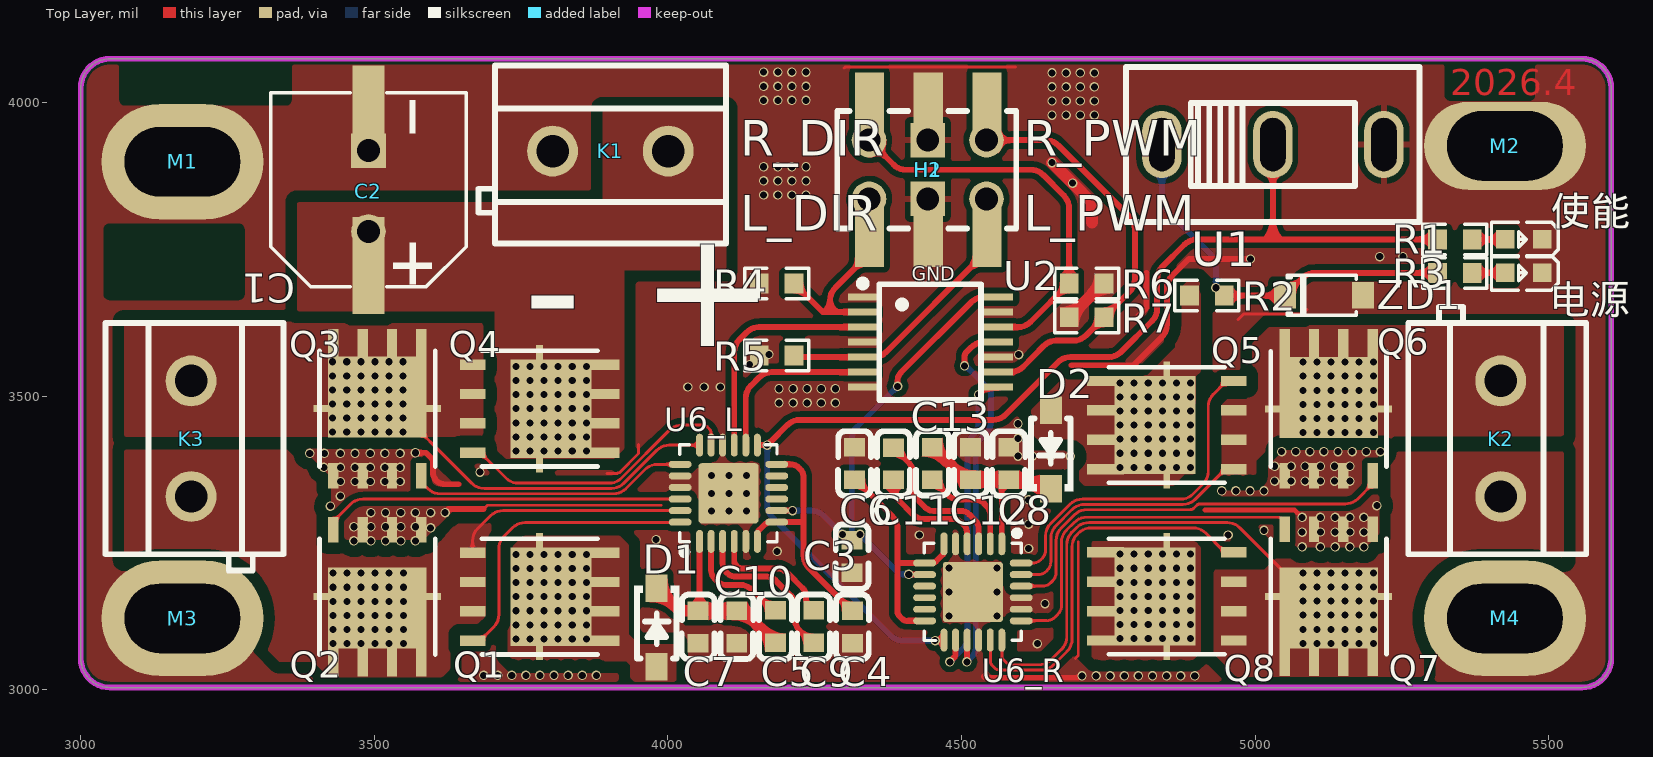
[diagram p0: Top Layer view]
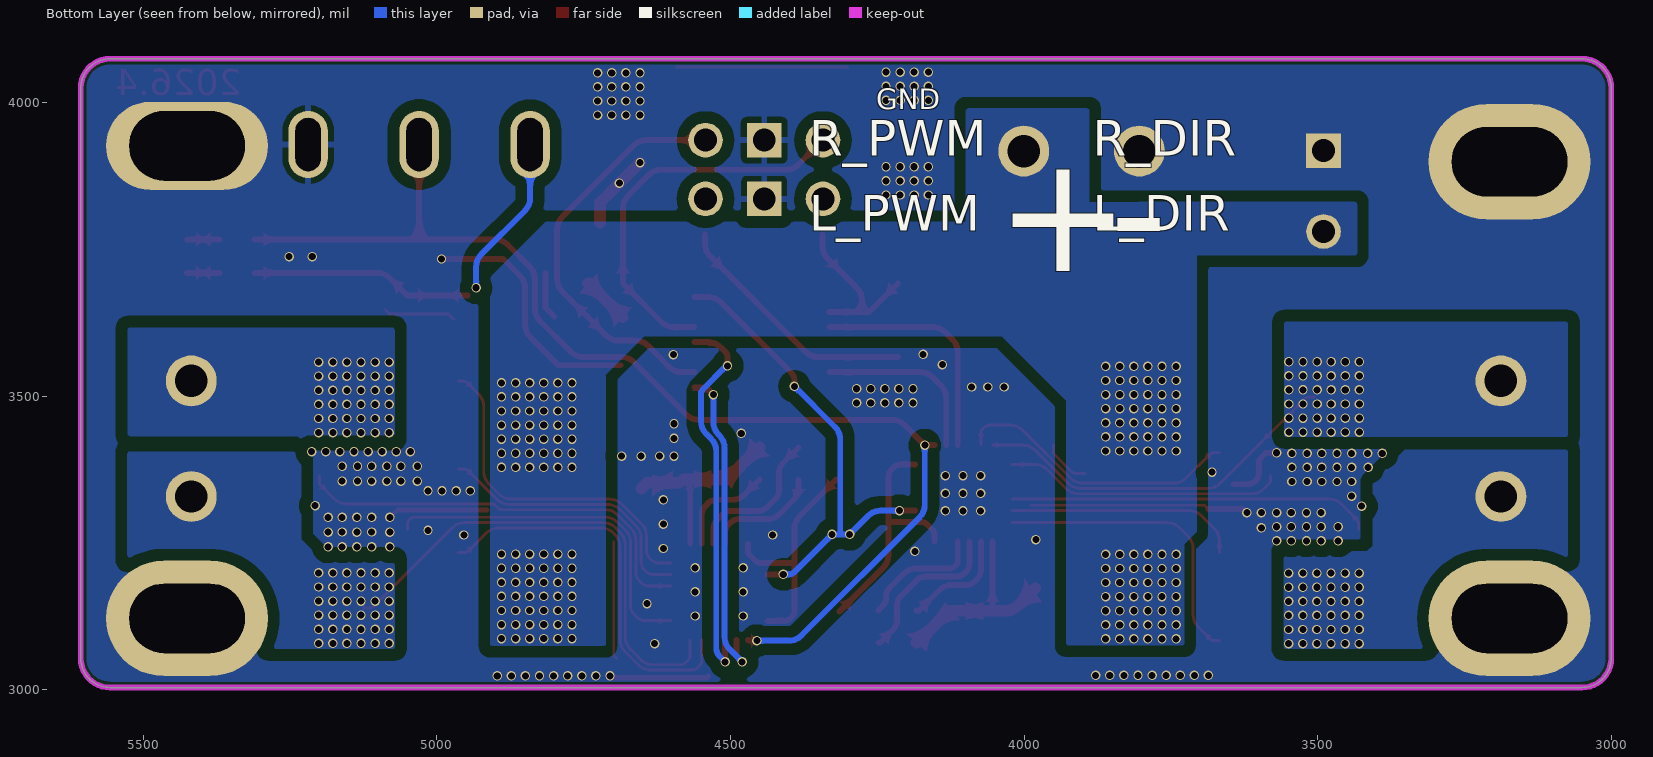
[diagram p1: Bottom Layer view, seen from below]
# Altium PCB MISC49921.pcbdoc (part 1 of 2)
Units mil, origin at the board's own origin, x right, y up, seen from the top; angles counter-clockwise.
Board outline 2606.3 x 1070.87 mil, 2 copper layers (Top Layer, Bottom Layer), stack 62.206 mil thick; 46 components, 37 nets, 219 pads, 514 vias.

## Layer stack, top to bottom
Top Solder Mask Layer: solder mask 0.394, Dk 3.3
Top Layer: signal copper 1.379
Dielectric1: surface 59.449, FR4, Dk 4.5
Bottom Layer: signal copper 1.378
Bottom Solder Mask Layer: solder mask 0.394, Dk 3.3

## Board outline
3050,4074.6 ccw(c3050,4024.6) 3000,4024.6 3000,3053.73 ccw(c3050,3053.73) 3050,3003.73 5556.3,3003.73 ccw(c5556.3,3053.73) 5606.3,3053.73 5606.3,4024.6 ccw(c5556.3,4024.6) 5556.3,4074.6

## Design rules (kind name [scope] priority, off if disabled: settings)
BoardOutlineClearance copperThickness2oz_1 [All] p2 off: genericclearance=8 ignorepadtopadclearanceinfootprint=FALSE except(0: Arc-SplitContinuation Track-SplitContinuation SMDPad-SplitContinuation THPad-SplitContinuation Via-SplitContinuation Fill-SplitContinuation Region-SplitContinuation Poly-SplitContinuation Text-SplitContinuation Hole-SplitContinuation; 6: Arc-CutoutEdge Track-CutoutEdge SMDPad-CutoutEdge THPad-CutoutEdge Via-CutoutEdge Text-CutoutEdge; 6.9: Hole-OutlineEdge Hole-CutoutEdge; 10: Poly-OutlineEdge Poly-CutoutEdge; 11.8: Arc-OutlineEdge Track-OutlineEdge SMDPad-OutlineEdge THPad-OutlineEdge Via-OutlineEdge Fill-OutlineEdge Region-OutlineEdge Text-OutlineEdge Fill-CutoutEdge Region-CutoutEdge)
BoardOutlineClearance Plane_innerPlane_1 [All] p4 off: genericclearance=4 ignorepadtopadclearanceinfootprint=FALSE except(0: Arc-SplitContinuation Track-SplitContinuation SMDPad-SplitContinuation THPad-SplitContinuation Via-SplitContinuation Fill-SplitContinuation Region-SplitContinuation Poly-SplitContinuation Text-SplitContinuation Hole-SplitContinuation; 6: Arc-CutoutEdge Track-CutoutEdge SMDPad-CutoutEdge THPad-CutoutEdge Via-CutoutEdge Text-CutoutEdge; 6.9: Hole-OutlineEdge Hole-CutoutEdge; 10: Poly-OutlineEdge Poly-CutoutEdge; 11.8: Arc-OutlineEdge Track-OutlineEdge SMDPad-OutlineEdge THPad-OutlineEdge Via-OutlineEdge Fill-OutlineEdge Region-OutlineEdge Text-OutlineEdge Fill-CutoutEdge Region-CutoutEdge)
BoardOutlineClearance Copper_copperRegion_1 [All] p6 off: genericclearance=4 ignorepadtopadclearanceinfootprint=FALSE except(0: Arc-SplitContinuation Track-SplitContinuation SMDPad-SplitContinuation THPad-SplitContinuation Via-SplitContinuation Fill-SplitContinuation Region-SplitContinuation Poly-SplitContinuation Text-SplitContinuation Hole-SplitContinuation; 6: Arc-CutoutEdge Track-CutoutEdge SMDPad-CutoutEdge THPad-CutoutEdge Via-CutoutEdge Text-CutoutEdge; 6.9: Hole-OutlineEdge Hole-CutoutEdge; 10: Poly-OutlineEdge Poly-CutoutEdge; 11.8: Arc-OutlineEdge Track-OutlineEdge SMDPad-OutlineEdge THPad-OutlineEdge Via-OutlineEdge Fill-OutlineEdge Region-OutlineEdge Text-OutlineEdge Fill-CutoutEdge Region-CutoutEdge)
BoardOutlineClearance Copper_直连_1 [All] p8 off: genericclearance=4 ignorepadtopadclearanceinfootprint=FALSE except(0: Arc-SplitContinuation Track-SplitContinuation SMDPad-SplitContinuation THPad-SplitContinuation Via-SplitContinuation Fill-SplitContinuation Region-SplitContinuation Poly-SplitContinuation Text-SplitContinuation Hole-SplitContinuation; 6: Arc-CutoutEdge Track-CutoutEdge SMDPad-CutoutEdge THPad-CutoutEdge Via-CutoutEdge Text-CutoutEdge; 6.9: Hole-OutlineEdge Hole-CutoutEdge; 10: Poly-OutlineEdge Poly-CutoutEdge; 11.8: Arc-OutlineEdge Track-OutlineEdge SMDPad-OutlineEdge THPad-OutlineEdge Via-OutlineEdge Fill-OutlineEdge Region-OutlineEdge Text-OutlineEdge Fill-CutoutEdge Region-CutoutEdge)
BoardOutlineClearance Copper_18_1 [All] p10 off: genericclearance=4 ignorepadtopadclearanceinfootprint=FALSE except(0: Arc-SplitContinuation Track-SplitContinuation SMDPad-SplitContinuation THPad-SplitContinuation Via-SplitContinuation Fill-SplitContinuation Region-SplitContinuation Poly-SplitContinuation Text-SplitContinuation Hole-SplitContinuation; 6: Arc-CutoutEdge Track-CutoutEdge SMDPad-CutoutEdge THPad-CutoutEdge Via-CutoutEdge Text-CutoutEdge; 6.9: Hole-OutlineEdge Hole-CutoutEdge; 10: Poly-OutlineEdge Poly-CutoutEdge; 11.8: Arc-OutlineEdge Track-OutlineEdge SMDPad-OutlineEdge THPad-OutlineEdge Via-OutlineEdge Fill-OutlineEdge Region-OutlineEdge Text-OutlineEdge Fill-CutoutEdge Region-CutoutEdge)
BoardOutlineClearance copperThickness1oz_1 [All] p12: genericclearance=4 ignorepadtopadclearanceinfootprint=FALSE except(0: Arc-SplitContinuation Track-SplitContinuation SMDPad-SplitContinuation THPad-SplitContinuation Via-SplitContinuation Fill-SplitContinuation Region-SplitContinuation Poly-SplitContinuation Text-SplitContinuation Hole-SplitContinuation; 6: Arc-CutoutEdge Track-CutoutEdge SMDPad-CutoutEdge THPad-CutoutEdge Via-CutoutEdge Text-CutoutEdge; 6.9: Hole-OutlineEdge Hole-CutoutEdge; 10: Poly-OutlineEdge Poly-CutoutEdge; 11.8: Arc-OutlineEdge Track-OutlineEdge SMDPad-OutlineEdge THPad-OutlineEdge Via-OutlineEdge Fill-OutlineEdge Region-OutlineEdge Text-OutlineEdge Fill-CutoutEdge Region-CutoutEdge)
Clearance copperThickness2oz [All] p1 off: gap=8 ignorepadtopadclearanceinfootprint=FALSE except(6: SMDPad-Track SMDPad-SMDPad THPad-Track SMDPad-THPad THPad-THPad Track-Via SMDPad-Via THPad-Via Via-Via Fill-SMDPad Region-SMDPad Fill-THPad Region-THPad Fill-Via Region-Via Arc-Track Arc-SMDPad Arc-THPad Arc-Via Fill-Arc Region-Arc Arc-Arc Text-Track SMDPad-Text Text-THPad Text-Via Fill-Text Region-Text Arc-Text Text-Text; 6.9: Hole-Track Hole-SMDPad Hole-THPad Hole-Via Fill-Hole Region-Hole Hole-Arc Hole-Text; 10: Poly-Track Poly-SMDPad Poly-THPad Poly-Via Poly-Fill Poly-Region Poly-Poly Poly-Arc Poly-Text Poly-Hole; 11.8: Fill-Track Region-Track; 20: Fill-Fill Fill-Region Region-Region)
Clearance Plane_innerPlane [All] p3 off: gap=4 ignorepadtopadclearanceinfootprint=FALSE except(6: SMDPad-Track SMDPad-SMDPad THPad-Track SMDPad-THPad THPad-THPad Track-Via SMDPad-Via THPad-Via Via-Via Fill-SMDPad Region-SMDPad Fill-THPad Region-THPad Fill-Via Region-Via Arc-Track Arc-SMDPad Arc-THPad Arc-Via Fill-Arc Region-Arc Arc-Arc Text-Track SMDPad-Text Text-THPad Text-Via Fill-Text Region-Text Arc-Text Text-Text; 6.9: Hole-Track Hole-SMDPad Hole-THPad Hole-Via Fill-Hole Region-Hole Hole-Arc Hole-Text; 10: Poly-Track Poly-SMDPad Poly-THPad Poly-Via Poly-Fill Poly-Region Poly-Poly Poly-Arc Poly-Text Poly-Hole; 11.8: Fill-Track Region-Track; 12: Fill-Fill Fill-Region Region-Region)
Clearance Copper_copperRegion [All] p5 off: gap=4 ignorepadtopadclearanceinfootprint=FALSE except(6: SMDPad-Track SMDPad-SMDPad THPad-Track SMDPad-THPad THPad-THPad Track-Via SMDPad-Via THPad-Via Via-Via Fill-SMDPad Region-SMDPad Fill-THPad Region-THPad Fill-Via Region-Via Arc-Track Arc-SMDPad Arc-THPad Arc-Via Fill-Arc Region-Arc Arc-Arc Text-Track SMDPad-Text Text-THPad Text-Via Fill-Text Region-Text Arc-Text Text-Text; 6.9: Hole-Track Hole-SMDPad Hole-THPad Hole-Via Fill-Hole Region-Hole Hole-Arc Hole-Text; 10: Poly-Track Poly-SMDPad Poly-THPad Poly-Via Poly-Fill Poly-Region Poly-Poly Poly-Arc Poly-Text Poly-Hole; 11.8: Fill-Track Region-Track; 12: Fill-Fill Fill-Region Region-Region)
Clearance Copper_直连 [All] p7 off: gap=4 ignorepadtopadclearanceinfootprint=FALSE except(6: SMDPad-Track SMDPad-SMDPad THPad-Track SMDPad-THPad THPad-THPad Track-Via SMDPad-Via THPad-Via Via-Via Fill-SMDPad Region-SMDPad Fill-THPad Region-THPad Fill-Via Region-Via Arc-Track Arc-SMDPad Arc-THPad Arc-Via Fill-Arc Region-Arc Arc-Arc Text-Track SMDPad-Text Text-THPad Text-Via Fill-Text Region-Text Arc-Text Text-Text; 6.9: Hole-Track Hole-SMDPad Hole-THPad Hole-Via Fill-Hole Region-Hole Hole-Arc Hole-Text; 10: Poly-Track Poly-SMDPad Poly-THPad Poly-Via Poly-Fill Poly-Region Poly-Poly Poly-Arc Poly-Text Poly-Hole; 11.8: Fill-Track Region-Track; 12: Fill-Fill Fill-Region Region-Region)
Clearance Copper_18 [All] p9 off: gap=4 ignorepadtopadclearanceinfootprint=FALSE except(6: SMDPad-Track SMDPad-SMDPad THPad-Track SMDPad-THPad THPad-THPad Track-Via SMDPad-Via THPad-Via Via-Via Fill-SMDPad Region-SMDPad Fill-THPad Region-THPad Fill-Via Region-Via Arc-Track Arc-SMDPad Arc-THPad Arc-Via Fill-Arc Region-Arc Arc-Arc Text-Track SMDPad-Text Text-THPad Text-Via Fill-Text Region-Text Arc-Text Text-Text; 6.9: Hole-Track Hole-SMDPad Hole-THPad Hole-Via Fill-Hole Region-Hole Hole-Arc Hole-Text; 11.8: Fill-Track Region-Track; 12: Fill-Fill Fill-Region Region-Region; 20: Poly-Track Poly-SMDPad Poly-THPad Poly-Via Poly-Fill Poly-Region Poly-Poly Poly-Arc Poly-Text Poly-Hole)
Clearance copperThickness1oz [All] p11: gap=4 ignorepadtopadclearanceinfootprint=FALSE except(6: SMDPad-Track SMDPad-SMDPad THPad-Track SMDPad-THPad THPad-THPad Track-Via SMDPad-Via THPad-Via Via-Via Fill-SMDPad Region-SMDPad Fill-THPad Region-THPad Fill-Via Region-Via Arc-Track Arc-SMDPad Arc-THPad Arc-Via Fill-Arc Region-Arc Arc-Arc Text-Track SMDPad-Text Text-THPad Text-Via Fill-Text Region-Text Arc-Text Text-Text; 6.9: Hole-Track Hole-SMDPad Hole-THPad Hole-Via Fill-Hole Region-Hole Hole-Arc Hole-Text; 10: Poly-Track Poly-SMDPad Poly-THPad Poly-Via Poly-Fill Poly-Region Poly-Poly Poly-Arc Poly-Text Poly-Hole; 11.8: Fill-Track Region-Track; 12: Fill-Fill Fill-Region Region-Region)
DiffPairsRouting differentialPair [All] p1: maxlimit=6 minlimit=6 mostfreqgap=6 toplayer_minwidth=5 toplayer_prefwidth=10 toplayer_maxwidth=100 toplayer_mingap=6 toplayer_prefgap=6 toplayer_maxgap=6 bottomlayer_minwidth=5 bottomlayer_prefwidth=10 bottomlayer_maxwidth=100 bottomlayer_mingap=6 bottomlayer_prefgap=6 bottomlayer_maxgap=6 maxuncoupledlength=10
HoleToHoleClearance otherClearance [All] p1: gap=11.8 allowstackedmicrovias=TRUE
Length netLength [All] p1: minlimit=0 maxlimit=0
PasteMaskExpansion pasteMaskExpansion [All] p1: expansion=0
PlaneConnect innerPlane [All] p1: planeconnectstyle=Relief reliefexpansion=20 reliefentries=4 reliefconductorwidth=10 reliefairgap=10
PolygonConnect 直连 [All] p1 off: connectstyle=Direct reliefconductorwidth=10 reliefentries=4 polygonreliefangle="90 Angle" airgapwidth=10 via.connectstyle=Relief via.reliefconductorwidth=10 via.reliefentries=4 via.polygonreliefangle="90 Angle" via.airgapwidth=10
PolygonConnect 18 [All] p2 off: connectstyle=Relief reliefconductorwidth=10 reliefentries=4 polygonreliefangle="90 Angle" airgapwidth=10 smdpad.connectstyle=Direct via.connectstyle=Relief via.reliefconductorwidth=10 via.reliefentries=4 via.polygonreliefangle="90 Angle" via.airgapwidth=10
PolygonConnect copperRegion [All] p3: connectstyle=Relief reliefconductorwidth=10 reliefentries=4 polygonreliefangle="90 Angle" airgapwidth=10 smdpad.connectstyle=Direct via.connectstyle=Relief via.reliefconductorwidth=10 via.reliefentries=4 via.polygonreliefangle="90 Angle" via.airgapwidth=10
RoutingVias viaSize [All] p1: holewidth=12 width=24 viastyle="Through Hole" minholewidth=11.8 minwidth=15.7 maxholewidth=248 maxwidth=393.7
SolderMaskExpansion solderMaskExpansion [IsVia] p1: expansion=-1000 istentingtop=TRUE
SolderMaskExpansion solderMaskExpansion [All] p2: expansion=2 istentingtop=FALSE
Width copperThickness2oz_2 [All] p1 off: maxlimit=100 minlimit=8 preferedwidth=10
Width copperThickness1oz_2 [All] p2: maxlimit=100 minlimit=5 preferedwidth=10

## Components (designator, comment, footprint, x,y, rotation, side; value= is the part's Value field where it differs from the comment)
C1 "220uF" CAP-SMD_BD8.0-L8.3-W8.3-FD 3490,3851.4 r90 top
C2 "220uF" CAP-TH_BD8.0-P3.50-D0.6-FD 3490,3849.19 r90 top
C3 "1UF" C0603 4313.61,3226.94 r90 top
C4 "1UF" C0603 4314.03,3106.95 r270 top
C5 "1UF" C0603 4183,3107.56 r90 top
C6 "1UF" C0603 4317.88,3385.6 r90 top
C7 "10UF" C0603 4051.33,3106.95 r270 top
C8 "10UF" C0603 4580.36,3385.6 r90 top
C9 "100nF" C0603 4248.12,3107.56 r90 top
C10 "100nF" C0603 4117.14,3106.95 r270 top
C11 "100nF" C0603 4383.79,3384.99 r270 top
C12 "100nF" C0603 4515.24,3385.6 r90 top
C13 "1UF" C0603 4450.12,3385.6 r270 top
D1 "1N5819W" SOD-123_L2.7-W1.6-LS3.7-RD-1 3980.81,3106.05 r270 top
D2 "1N5819W" SOD-123_L2.7-W1.6-LS3.7-RD-1 4651.88,3409.05 r90 top
H1 "贴片" HDR-SMD_6P-P2.54-V-M-R2-C5-S7.4 4443.16,3885.68 r0 top locked
H2 "" HDR-TH_6P-P2.54-V-R2-C3-S2.54_A2541WV-2X3P 4442.39,3885.88 r0 top locked
K1 "KF301-5.0-2P" CONN-TH_P5.00_KF301-5.0-2P 3902,3917.23 r180 top
K2 "KF301-5.0-2P" CONN-TH_P5.00_KF301-5.0-2P 5418,3427.56 r90 top
K3 "KF301-5.0-2P" CONN-TH_P5.00_KF301-5.0-2P 3188,3427.56 r270 top
M1 "" M4螺丝#1 3173.23,3899.12 r0 top
M2 "" M4螺丝#2 5425.2,3926.25 r0 top
M3 "" M4螺丝#1 3173.23,3121.56 r0 top
M4 "" M4螺丝#1 5425.2,3121.56 r0 top
Q1 "TPH1R403NL" DFN5x6 3781.49,3158.6 r270 top
Q2 "TPH1R403NL" DFN5x6 3505,3158.6 r180 top
Q3 "TPH1R403NL" DFN5x6 3505,3478.6 r0 top
Q4 "TPH1R403NL" DFN5x6 3781.49,3478.6 r270 top
Q5 "TPH1R403NL" DFN5x6 4849.3,3450.76 r90 top
Q6 "TPH1R403NL" DFN5x6 5125,3478.32 r0 top
Q7 "TPH1R403NL" DFN5x6 5125,3158.96 r180 top
Q8 "TPH1R403NL" DFN5x6 4849.3,3158.96 r90 top
R1 "2.2K" R0603 5340,3766.89 r180 top
R2 "2.2K" R0603 4917.65,3671.08 r180 top
R3 "2.2K" R0603 5340,3709.87 r180 top
R4 "10K" R0603 4185,3692.07 r180 top
R5 "10K" R0603 4185,3569.37 r180 top
R6 "10K" R0603 4712.79,3692.07 r180 top
R7 "10K" R0603 4712.79,3634.37 r0 top
U1 "SS12D10G5" SW-TH_SHOU-HAN_SS12D10G4 5030,3928.47 r0 top
U2 "SN74HC125PWR" TSSOP-14_L5.0-W4.4-P0.65-LS6.5-BL 4446.48,3592.03 r270 top
U6_L "DRV8701ERGET" VQFN-24_L4.0-W4.0-P0.50-BL-EP2.5 4103,3334.6 r0 top
U6_R "DRV8701ERGET" VQFN-24_L4.0-W4.0-P0.50-BL-EP2.5 4519.24,3166.6 r180 top
ZD1 "BZT52C3V6" SOD-123_L2.8-W1.8-LS3.7-RD 5117,3671.48 r0 top
使能 "" LED_0603 5455,3766.79 r180 top
电源 "" LED_0603 5455,3709.77 r180 top

## Footprints (in the part's own frame and the unit in brackets; to place one, negate y for a bottom-side part, rotate by r counter-clockwise, add the part's x,y. Pads: shape width x height; smd on the part's side, far side on the other; paste and mask are expansions set on the pad)
C0603 [mm]
  rect 0.8x0.9 smd: 1(-0.7,0) 2(0.7,0)
  silkscreen extent -1.41,-0.71 1.39,0.72
CAP-SMD_BD8.0-L8.3-W8.3-FD [mm]
  rect 4.2x1.4 smd: 1(-3.267,0) 2(3.267,0)
  silkscreen extent -4.2,-4.23 4.2,4.23
CAP-TH_BD8.0-P3.50-D0.6-FD [mil]
  round 59 hole 39: 1(-68.9,0)
  rect 59x59 hole 39: 2(68.9,0)
CONN-TH_P5.00_KF301-5.0-2P [mm]
  round 2.2 hole 1.4: 1(-2.5,0) 2(2.5,0)
  silkscreen extent -5,-3.7 5.71,4
DFN5x6 [mm]
  rect 0.45x1.6 smd: 1(-1.905,2.65) 1(-0.635,2.65) 1(0.635,2.65) 1(1.905,2.65)
  rect 5.5x0.3 smd: 1(0,0)
  rect 4.25x3.5 smd: 1(0,0.5)
  rect 0.45x1.1 smd: 2(1.905,-2.9) 3(-1.905,-2.9) 3(-0.635,-2.9) 3(0.635,-2.9)
  silkscreen extent -2.5,-2.5 2.5,2.5
HDR-SMD_6P-P2.54-V-M-R2-C5-S7.4 [mm]
  rect 1.27x2.8 smd: 1(-2.54,-2.8) 2(-2.54,2.8) 3(0,-2.8) 4(0,2.8) 5(2.54,-2.8) 6(2.54,2.8)
  silkscreen extent -3.94,-2.54 3.81,2.54
HDR-TH_6P-P2.54-V-R2-C3-S2.54_A2541WV-2X3P [mil]
  round 59 hole 39: 1(-100,-50) 2(-100,50) 5(100,-50) 6(100,50)
  rect 59x59 hole 39: 3(0,-50) 4(0,50)
LED_0603 [mil]
  rect 31.5x31.5 smd paste+0 mask+2: 1(-33.5,-0.4) 2(29.5,-0.2)
  silkscreen extent -61,-30 53,30
M4螺丝#1 [mm]
  oval 7x5 hole 3 slot 5 at 0 deg paste+0 mask+0.127: 1(0,0)
M4螺丝#2 [mm]
  oval 7x3.81 hole 3 slot 5 at 0 deg paste+0 mask+0.127: 1(0,0)
R0603 [mil]
  rect 31.75x34.02 smd paste-3937.01 mask+2: 1(-29.66,0) 2(29.66,0)
  silkscreen extent -55,-26 55,26
SOD-123_L2.7-W1.6-LS3.7-RD-1 [mm]
  rect 1.2x0.95 smd: 1(-1.7,0) 2(1.7,0)
  silkscreen extent -1.81,-0.98 1.35,0.98
SOD-123_L2.8-W1.8-LS3.7-RD [mm]
  rect 0.95x1.15 smd: 1(-1.692,0) 2(1.692,0)
  silkscreen extent -1.58,-0.87 1.41,0.87
SW-TH_SHOU-HAN_SS12D10G4 [mm]
  oval 1.7x2.9 hole 1.1 slot 2.3 at 90 deg paste+0 mask+0.05: 1(-4.8,0) 2(0,0) 3(4.8,0)
  silkscreen extent -6.35,-3.35 6.35,3.35
TSSOP-14_L5.0-W4.4-P0.65-LS6.5-BL [mil]
  rect 12x50 smd paste+0 mask+1.97: 1(-76.77,-115.16) 2(-51.18,-115.16) 3(-25.59,-115.16) 4(0,-115.16) 5(25.59,-115.16) 6(51.18,-115.16) 7(76.77,-115.16) 8(76.77,116.16) 9(51.18,116.16) 10(25.59,116.16) 11(0,116.16) 12(-25.59,116.16) 13(-51.18,116.16) 14(-76.77,116.16)
  silkscreen extent -106,-121 98,87
VQFN-24_L4.0-W4.0-P0.50-BL-EP2.5 [mil]
  rrect100% 11.81x39 smd paste-3937 mask+2: 1(-49.21,-81.95) 2(-29.53,-81.95) 3(-9.84,-81.95) 4(9.84,-81.95) 5(29.53,-81.95) 6(49.21,-81.95) 13(49.21,81.96) 14(29.53,81.96) 15(9.84,81.96) 16(-9.84,81.96) 17(-29.53,81.96) 18(-49.21,81.96)
  rrect100% 39x11.81 smd paste-3937 mask+2: 7(82.2,-49.21) 8(82.2,-29.52) 9(82.2,-9.84) 10(82.2,9.84) 11(82.2,29.53) 12(82.2,49.21) 19(-82.2,49.21) 20(-82.2,29.53) 21(-82.2,9.84) 22(-82.2,-9.84) 23(-82.2,-29.52) 24(-82.2,-49.21)
  rrect10% 102.36x102.36 smd paste-3937 mask+2: 25(0.03,-0.03)
  silkscreen extent -83,-105 83,83

## Via types
v1: diameter 16, hole 12, Top Layer to Bottom Layer, 514 vias

## Nets (pads, with @x,y where several pads share a name; then routed paths per layer and width w, separated by ;. In a path a pad name is that pad's centre, name@x,y a point inside that pad or via, vN(x,y) a via of type N, cw(c..) or ccw(c..) an arc to the next point about the centre after c; other vN are vias at no path point)
3V6: R2.1 R3.2 U1.1 ZD1.1 | length 657.2
  Top Layer w10: R2.1@4947.31,3671.08 5049.98,3671.08 ZD1.1@5050.37,3671.48 5079.98,3701.09 cw(c5101.19,3679.87) 5101.19,3709.87 R3.2@5310.34,3709.87
  Bottom Layer w10: 4841.02,3837 U1.1@4841.02,3928.47 ; 4841.03,3837 ccw(c4871.02,3837) 4849.81,3815.79 4924.21,3741.39 cw(c4903,3720.17) 4933,3720.17 v1(4933,3684.6)
$1N440: R1.1 使能.2 | length 55.9
  Top Layer w10: R1.1@5369.66,3766.89 5425.4,3766.89 使能.2@5425.5,3766.99
$1N595: R3.1 电源.2 | length 55.9
  Top Layer w10: R3.1@5369.66,3709.87 5369.76,3709.97 电源.2@5425.5,3709.97
$1N3022: C9.1 U6_L.3 | length 274.9
  Top Layer w10: U6_L.3@4093.16,3252.65 4093.16,3214.73 ccw(c4113.16,3214.73) 4099.02,3200.58 4101.14,3198.46 ccw(c4115.28,3212.6) 4115.28,3192.6 4168.72,3192.6 cw(c4168.72,3172.6) 4182.86,3186.74 4210.14,3159.46 cw(c4196,3145.32) 4216,3145.32 4216,3121.47 ccw(c4246,3121.47) 4224.79,3100.26 4245.04,3080 C9.1@4248.12,3080
$1N3052: C9.2 U6_L.4 | length 213.4
  Top Layer w10: U6_L.4@4112.84,3252.65 4112.84,3219.35 ccw(c4122.84,3219.35) 4115.77,3212.27 4118.48,3209.56 ccw(c4125.55,3216.63) 4125.55,3206.63 4183.54,3206.63 cw(c4183.54,3176.63) 4204.76,3197.84 4229.14,3173.46 cw(c4215,3159.32) 4235,3159.32 4235,3156.53 ccw(c4255,3156.53) 4240.86,3142.38 C9.2@4248.12,3135.12
$1N3247: C5.2 U6_L.2 | length 188.9
  Top Layer w10: U6_L.2@4073.47,3252.65 4073.47,3203.42 ccw(c4093.47,3203.42) 4079.33,3189.27 4084.14,3184.46 ccw(c4098.28,3198.6) 4098.28,3178.6 4122.57,3178.6 cw(c4122.57,3148.6) 4143.79,3169.81 4178.48,3135.12 C5.2@4183,3135.12
$1N3253: C5.1 C7.1 C10.1 D1.1 U6_L.1 | length 358.7
  Top Layer w10: C7.1@4051.33,3134.51 4053.79,3136.97 U6_L.1@4053.79,3252.65
  Top Layer w20: D1.1@3980.81,3172.98 4010.49,3143.3 ccw(c4031.7,3164.51) 4031.7,3134.51 C7.1@4051.33,3134.51 C10.1@4117.14,3134.51 4124.35,3134.51 cw(c4124.35,3124.51) 4131.42,3131.58 4149.3,3113.7 4149.3,3112.75 4158.66,3103.39 4159.61,3103.39 C5.1@4183,3080
$1N4029: C11.1 U6_R.3 | length 256.8
  Top Layer w10: C11.1@4383.79,3412.55 4411.14,3385.19 cw(c4397,3371.05) 4417,3371.05 4417,3339.81 ccw(c4437,3339.81) 4422.86,3325.67 4438.07,3310.46 ccw(c4452.21,3324.6) 4452.21,3304.6 4498.72,3304.6 cw(c4498.72,3284.6) 4512.86,3298.74 4523.22,3288.38 cw(c4509.08,3274.24) 4529.08,3274.24 U6_R.3@4529.08,3248.55
$1N4031: C11.2 U6_R.4 | length 197
  Top Layer w10: C11.2@4383.79,3357.43 4383.79,3344.24 ccw(c4413.79,3344.24) 4392.58,3323.03 4416.21,3299.39 ccw(c4437.43,3320.6) 4437.43,3290.6 4485.72,3290.6 cw(c4485.72,3270.6) 4499.86,3284.74 4503.54,3281.06 cw(c4489.4,3266.92) 4509.4,3266.92 U6_R.4@4509.4,3248.55
$1N4034: C13.2 U6_R.2 | length 175.1
  Top Layer w10: C13.2@4450.12,3358.04 4475.77,3332.39 ccw(c4496.98,3353.6) 4496.98,3323.6 4523.72,3323.6 cw(c4523.72,3303.6) 4537.86,3317.74 4542.91,3312.69 cw(c4528.77,3298.55) 4548.77,3298.55 U6_R.2@4548.77,3248.55
$1N4036: C8.1 C12.1 C13.1 D2.1 U6_R.1 | length 335.5
  Top Layer w10: U6_R.1@4568.45,3248.55 4568.45,3337.84 cw(c4588.45,3337.84) 4574.31,3351.98 C8.1@4580.36,3358.04
  Top Layer w20: C13.1@4450.12,3413.16 4473.51,3389.77 4474.46,3389.77 4483.82,3380.4 4483.82,3379.45 4502.31,3360.96 ccw(c4509.38,3368.04) 4509.38,3358.04 C12.1@4515.24,3358.04 C8.1@4580.36,3358.04 ; C8.1@4586.96,3352.44 D2.1@4642.56,3352.44 ; D2.1@4642.56,3351.44 D2.1@4651.88,3342.12
AVDD_L: C4.1 U6_L.6 U6_L.7 U6_L.12 | length 420.9
  Top Layer w10: U6_L.6@4152.21,3252.65 4152.21,3264.71 cw(c4162.21,3264.71) 4155.14,3271.78 4165.82,3282.46 cw(c4172.89,3275.39) 4172.89,3285.39 U6_L.7@4185.2,3285.39 4229.01,3285.39 4230.98,3287.36 ; U6_L.12@4185.2,3383.81 4208.51,3383.81 cw(c4208.51,3363.81) 4222.65,3377.95 4225.13,3375.47 cw(c4210.98,3361.33) 4230.98,3361.33 4230.98,3287.36 ; C4.1@4314.03,3133.51 4239.77,3207.77 cw(c4260.98,3228.98) 4230.98,3228.98 4230.98,3287.36
AVDD_R: C6.1 U6_R.6 U6_R.7 U6_R.12 | length 410.4
  Top Layer w10: C6.1@4317.88,3358.04 4319.56,3358.04 4382.23,3295.37 cw(c4361.02,3274.16) 4391.02,3274.16 4391.02,3215.81 ; U6_R.12@4437.04,3117.39 4406.35,3117.39 cw(c4406.35,3127.39) 4399.28,3120.32 4393.94,3125.66 cw(c4401.02,3132.73) 4391.02,3132.73 4391.02,3215.81 ; U6_R.6@4470.03,3248.55 4470.03,3236.49 cw(c4460.03,3236.49) 4467.1,3229.42 4456.42,3218.74 cw(c4449.35,3225.81) 4449.35,3215.81 U6_R.7@4437.04,3215.81 4391.02,3215.81
D3V3: C3.2 U2.14 U6_L.8 U6_R.8 | length 819.5
  Top Layer w10: U6_L.8@4185.2,3305.08 v1(4212,3305.08) ; v1(4391,3516.6) 4391,3526.32 cw(c4411,3526.32) 4396.86,3540.46 4516.41,3660.01 cw(c4537.62,3638.8) 4537.62,3668.8 U2.14@4561.64,3668.8 ; v1(4410,3196.6) 4410.48,3196.12 U6_R.8@4437.04,3196.12
  Bottom Layer w10: v1(4212,3305.08) 4244.1,3305.08 cw(c4244.1,3275.08) 4265.31,3296.29 4294.07,3267.53 ccw(c4301.14,3274.6) 4301.14,3264.6 4313,3264.6 ; v1(4391,3516.6) 4321.79,3447.39 ccw(c4343,3426.17) 4313,3426.17 4313,3264.6 ; v1(4410,3196.6) 4399.14,3196.6 cw(c4399.14,3206.6) 4392.07,3199.53 4329.93,3261.67 ccw(c4322.86,3254.6) 4322.86,3264.6 4313,3264.6
  other v1: 4297,3264.6 4327,3264.6
GH1_L: Q4.2 U6_L.17 | length 491.9
  Top Layer w5: Q4.2@3667.31,3403.6 3676.86,3403.6 cw(c3676.86,3393.6) 3683.93,3400.67 3724.01,3360.59 ccw(c3745.22,3381.8) 3745.22,3351.8 3899.78,3351.8 ccw(c3899.78,3381.8) 3920.99,3360.59 4002.21,3441.81 cw(c4023.43,3420.6) 4023.43,3450.6 4059.86,3450.6 cw(c4059.86,3440.6) 4066.93,3447.67 4070.54,3444.06 cw(c4063.47,3436.99) 4073.47,3436.99 U6_L.17@4073.47,3416.56
GH1_R: Q8.2 U6_R.17 | length 675.5
  Top Layer w5: U6_R.17@4548.77,3084.64 4549,3084.41 4549,3048.74 ccw(c4559,3048.74) 4551.93,3041.67 4557.07,3036.53 ccw(c4564.14,3043.6) 4564.14,3033.6 4635.32,3033.6 ccw(c4635.32,3063.6) 4656.54,3042.39 4679.26,3065.11 ccw(c4658.05,3086.32) 4688.05,3086.32 4688.05,3243.29 cw(c4718.05,3243.29) 4696.83,3264.51 4699.26,3266.93 cw(c4720.47,3245.71) 4720.47,3275.71 4894.46,3275.71 cw(c4894.46,3245.71) 4915.67,3266.93 4945.71,3236.89 ccw(c4952.78,3243.96) 4952.78,3233.96 Q8.2@4963.47,3233.96
GH2_L: Q1.2 U6_L.24 | length 513
  Top Layer w5: Q1.2@3667.31,3083.6 3675.86,3083.6 ccw(c3675.86,3093.6) 3682.93,3086.53 3703.21,3106.81 ccw(c3682,3128.03) 3712,3128.03 3712,3240.17 cw(c3742,3240.17) 3720.79,3261.39 3735.21,3275.81 cw(c3756.43,3254.6) 3756.43,3284.6 4020.01,3284.6 U6_L.24@4020.8,3285.39
GH2_R: Q5.2 U6_R.24 | length 587.3
  Top Layer w5: U6_R.24@4601.44,3215.81 4620.93,3215.81 ccw(c4620.93,3235.81) 4635.07,3221.67 4637.11,3223.71 ccw(c4622.97,3237.85) 4642.97,3237.85 4642.97,3261.96 cw(c4672.97,3261.96) 4651.76,3283.18 4684.39,3315.81 cw(c4705.6,3294.6) 4705.6,3324.6 4872.82,3324.6 ccw(c4872.82,3354.6) 4894.04,3333.39 4911.21,3350.56 ccw(c4890,3371.78) 4920,3371.78 4920,3482.17 cw(c4950,3482.17) 4928.79,3503.39 4948.23,3522.83 cw(c4955.3,3515.76) 4955.3,3525.76 Q5.2@4963.47,3525.76
GL1_L: Q3.2 U6_L.19 | length 476.3
  Top Layer w5: Q3.2@3580,3364.43 3580,3357.74 ccw(c3590,3357.74) 3582.93,3350.67 3591.04,3342.56 ccw(c3612.25,3363.77) 3612.25,3333.77 3907.25,3333.77 ccw(c3907.25,3363.77) 3928.46,3342.56 3960.92,3375.02 cw(c3982.13,3353.81) 3982.13,3383.81 U6_L.19@4020.8,3383.81
GL1_R: Q7.2 U6_R.19 | length 608.2
  Top Layer w5: U6_R.19@4601.44,3117.39 4601.65,3117.6 4644.72,3117.6 ccw(c4644.72,3137.6) 4658.86,3123.46 4664.16,3128.76 ccw(c4650.02,3142.9) 4670.02,3142.9 4670.02,3250.76 cw(c4700.02,3250.76) 4678.8,3271.97 4691.79,3284.96 cw(c4713,3263.75) 4713,3293.75 5038.71,3293.75 cw(c5038.71,3283.75) 5045.78,3290.82 5047.07,3289.53 cw(c5040,3282.46) 5050,3282.46 Q7.2@5050,3273.14
GL2_L: Q2.2 U6_L.22 | length 618.7
  Top Layer w5: Q2.2@3430,3272.77 3430,3282.46 cw(c3440,3282.46) 3432.93,3289.53 3459.37,3315.97 cw(c3480.58,3294.76) 3480.58,3324.76 U6_L.22@4020.8,3324.76
GL2_R: Q6.2 U6_R.22 | length 721.5
  Top Layer w5: U6_R.22@4601.44,3176.44 4637.56,3176.44 ccw(c4637.56,3196.44) 4651.7,3182.3 4655.14,3185.74 ccw(c4641,3199.88) 4661,3199.88 4661,3254.5 cw(c4691,3254.5) 4669.79,3275.71 4691.89,3297.81 cw(c4713.1,3276.6) 4713.1,3306.6 4888.59,3306.6 ccw(c4888.59,3316.6) 4895.66,3309.53 4899.8,3313.67 cw(c4906.87,3306.6) 4906.87,3316.6 5153.57,3316.6 ccw(c5153.57,3346.6) 5174.79,3325.39 5197.07,3347.67 ccw(c5190,3354.74) 5200,3354.74 Q6.2@5200,3364.15
GND: C1.2 C2.2 C3.1 C4.2 C6.2 C7.2 C8.2 C10.2 C12.2 H1.3 H1.4 H2.3 H2.4 K1.2 M1.1 M2.1 M3.1 M4.1 Q2.3 Q3.3 Q6.3 Q7.3 R4.2 R5.2 R6.1 R7.1 U1.3 U2.1 U2.4 U2.7 U2.10 U2.13 U6_L.5 U6_L.16 U6_L.20 U6_L.21 U6_L.25 U6_R.5 U6_R.16 U6_R.20 U6_R.21 U6_R.25 ZD1.2 使能.1 电源.1 | length 2245.3
  Top Layer w5: 3686.13,3307.6 3692.78,3314.25 3988.49,3314.25 ; 3896,3368.6 3914.01,3368.6 3915,3369.59 3917.26,3369.59 3950,3402.33 3950,3417.6 ; 4300,4058.6 4301.7,4060.3 4592,4060.3 ; 4694,3053.6 4698.65,3058.25 4698.65,3251.33 ; 4971,3630.6 4979.98,3639.58 5079.98,3639.58 5088,3647.6
  Top Layer w8: 4914,3306.1 5067.5,3306.1 v1(5080,3293.6)
  Top Layer w10: v1(3570,3403.6) 3588,3403.6 3596.93,3394.67 cw(c3589.86,3387.6) 3599.86,3387.6 3599.86,3370.01 ccw(c3619.86,3370.01) 3619.86,3350.01 3643,3350.01 ; v1(3620.54,3301.6) 3626.54,3307.6 3686.13,3307.6 ; 4538,3022.6 4540.07,3020.53 4694.79,3020.53 ccw(c4694.79,3030.53) 4701.86,3023.46 4704.86,3023.46 v1(4705,3023.6) ; 4687,3552.6 4793,3552.6 4840.78,3600.38 ccw(c4819.57,3621.6) 4849.57,3621.6 4849.57,3683.74 cw(c4879.57,3683.74) 4858.36,3704.96 4887,3733.6 v1(4992,3733.6) ; 4800,3635.6 4815,3650.6 4815,3709.6
  Top Layer w20: v1(4654,3897.6) v1(4689,3862.6) 4722,3829.6 4722,3795.6 ; R7.1@4683.13,3634.37 4740.84,3692.07 R6.1@4742.45,3692.07
  other v1: 4729,3023.6 4753,3023.6 4777,3023.6 4801,3023.6 4825,3023.6 4849,3023.6 4873,3023.6 4897,3023.6 3686,3024.6 3710,3024.6 3734,3024.6 3758,3024.6 3782,3024.6 3806,3024.6 3830,3024.6 3854,3024.6 3878,3024.6 4629,3078.6 4478.27,3125.69 4560.16,3125.69 4642,3146.6 4478.27,3166.63 4560.16,3166.63 4478.27,3207.58 4560.16,3207.58 4186,3235.6 4614,3240.6 5080,3243.34 5111,3243.47 5136,3243.34 5161,3243.47 5185,3243.34 3465,3253.6 3494,3253.6 3519,3253.6 3545,3253.6 3570,3253.6 3980,3255.6 4428,3263.6 4954,3263.6 5080,3268.47 5136,3268.47 5185,3268.47 5111,3268.6 5161,3268.6 5015,3271.6 3596,3275.6 3465,3277.6 3494,3277.6 3519,3277.6 3545,3277.6 3570,3277.6 4614,3281.96 5111,3293.73 5136,3293.6 5161,3293.73 5185,3293.6 3494,3301.6 3519,3301.6 3545,3301.6 3570,3301.6 3596,3301.6 4074,3304.6 4104,3304.6 4134,3304.6 3425,3312.6 5207,3313.6 4614,3323.32 3442,3329.6 4074,3334.6 4104,3334.6 4134,3334.6 4943,3338.6 4967,3338.6 4991,3338.6 5015,3338.6 3442,3354.6 3467,3354.6 3493,3354.6 3518,3354.6 3544,3354.6 5033,3355.25 5061,3355.25 5085,3355.25 5111,3355.25 5135,3355.25 5161,3355.25 4074,3364.6 4104,3364.6 4134,3364.6 3680,3370.6 3414,3378.6 3442,3378.6 3467,3378.6 3493,3378.6 3518,3378.6 3544,3378.6 5033,3380.6 5061,3380.6 5085,3380.6 5111,3380.6 5135,3380.6 5161,3380.6 4596.12,3397.73 4620.39,3397.73 4651.88,3397.73 4685.19,3397.73 3390,3402.6 3415,3402.6 3442,3402.6 3467,3402.6 3493,3402.6 3518,3402.6 3544,3402.6 5045,3405.6 5069,3405.6 5093,3405.6 5117,3405.6 5141,3405.6 5165,3405.6 5189,3405.6 5213,3405.6 4596.12,3428.12 4481.5,3436.75 4596.12,3453.03 4189,3488.6 4213,3488.6 4237,3488.6 4261,3488.6 4285,3488.6 4189,3512.6 4213,3512.6 4237,3512.6 4261,3512.6 4285,3512.6 4034,3515.6 4061.56,3515.6 4089.12,3515.6 4139,3553.6 4171.93,3571.11 4597,3570.6 5212,3737.6 5251.32,3737.6 4163,3842.6 4187,3842.6 4211,3842.6 4235,3842.6 4163,3866.6 4187,3866.6 4211,3866.6 4235,3866.6 4163,3890.6 4187,3890.6 4211,3890.6 4235,3890.6 4654,3978.6 4678,3978.6 4702,3978.6 4726,3978.6 4654,4002.6 4678,4002.6 4702,4002.6 4726,4002.6 4163,4003.6 4187,4003.6 4211,4003.6 4235,4003.6 4654,4026.6 4678,4026.6 4702,4026.6 4726,4026.6 4163,4027.6 4187,4027.6 4211,4027.6 4235,4027.6 4654,4050.6 4678,4050.6 4702,4050.6 4726,4050.6 4163,4051.6 4187,4051.6 4211,4051.6 4235,4051.6
L_A: K3.2 Q1.3 Q2.1 U6_L.23 | length 399.4
  Top Layer w5: Q1.3@3667.31,3233.6 3667.31,3253.49 cw(c3697.31,3253.49) 3676.1,3274.7 3697.69,3296.29 cw(c3718.9,3275.08) 3718.9,3305.08 U6_L.23@4020.8,3305.08
  other v1: 3429.35,3078.6 3453.35,3078.6 3477.35,3078.6 3501.35,3078.6 3525.35,3078.6 3549.35,3078.6 3429.35,3102.6 3453.35,3102.6 3477.35,3102.6 3501.35,3102.6 3525.35,3102.6 3549.35,3102.6 3429.35,3126.6 3453.35,3126.6 3477.35,3126.6 3501.35,3126.6 3525.35,3126.6 3549.35,3126.6 3429.35,3150.6 3453.35,3150.6 3477.35,3150.6 3501.35,3150.6 3525.35,3150.6 3549.35,3150.6 3429.35,3174.6 3453.35,3174.6 3477.35,3174.6 3501.35,3174.6 3525.35,3174.6 3549.35,3174.6 3429.35,3198.6 3453.35,3198.6 3477.35,3198.6 3501.35,3198.6 3525.35,3198.6 3549.35,3198.6
L_B: K3.1 Q3.1 Q4.3 U6_L.18 | length 639.5
  Top Layer w5: Q3.1@3505,3498.29 3515.17,3498.29 cw(c3515.17,3488.29) 3522.24,3495.36 3666.03,3351.57 ccw(c3687.24,3372.79) 3687.24,3342.79 3903.51,3342.79 ccw(c3903.51,3372.79) 3924.72,3351.57 3980.92,3407.77 cw(c4002.13,3386.56) 4002.13,3416.56 U6_L.18@4053.79,3416.56
  other v1: 3429,3438.6 3453,3438.6 3477,3438.6 3501,3438.6 3525,3438.6 3549,3438.6 3429,3462.6 3453,3462.6 3477,3462.6 3501,3462.6 3525,3462.6 3549,3462.6 3429,3486.6 3453,3486.6 3477,3486.6 3501,3486.6 3525,3486.6 3549,3486.6 3429,3510.6 3453,3510.6 3477,3510.6 3501,3510.6 3525,3510.6 3549,3510.6 3429,3534.6 3453,3534.6 3477,3534.6 3501,3534.6 3525,3534.6 3549,3534.6 3429,3558.6 3453,3558.6 3477,3558.6 3501,3558.6 3525,3558.6 3549,3558.6
L_DIR_IN: H1.1 H2.1 R4.1 U2.2 | length 294.4
  Top Layer w10: R4.1@4214.66,3692.07 4263.53,3643.21 4275.95,3643.21 ; U2.2@4331.32,3643.21 4275.95,3643.21 ; H1.1@4343.16,3775.44 4343.16,3755.18 cw(c4313.16,3755.18) 4334.37,3733.97 4284.74,3684.34 ccw(c4305.95,3663.13) 4275.95,3663.13 4275.95,3643.21
L_DIR_O: U2.3 U6_L.15 | length 399.3
  Top Layer w10: U6_L.15@4112.84,3416.56 4112.84,3575.01 cw(c4142.84,3575.01) 4121.63,3596.23 4134.23,3608.83 cw(c4155.44,3587.62) 4155.44,3617.62 U2.3@4331.32,3617.62
L_PWM_IN: H1.5 H2.5 R5.1 U2.5 | length 429.2
  Top Layer w10: R5.1@4214.73,3566.44 U2.5@4331.32,3566.44 4350.41,3566.44 ccw(c4350.41,3596.44) 4371.62,3575.22 4534.37,3737.97 ccw(c4513.16,3759.18) 4543.16,3759.18 H1.5@4543.16,3775.44
L_PWM_O: U2.6 U6_L.14 | length 301.9
  Top Layer w10: U6_L.14@4132.53,3416.56 4132.53,3496.7 cw(c4162.53,3496.7) 4141.32,3517.92 4155.46,3532.06 cw(c4176.67,3510.85) 4176.67,3540.85 U2.6@4331.32,3540.85
PWR_EN: R1.2 U1.2 U6_L.13 U6_R.13 | length 2002.7
  Top Layer w10: U6_L.13@4152.25,3416.6 4160.72,3416.6 ccw(c4160.72,3436.6) 4168.37,3418.12 ccw(c4160.72,3436.6) 4174.86,3422.46 4203.21,3450.81 cw(c4224.43,3429.6) 4224.43,3459.6 4553.57,3459.6 ccw(c4553.57,3489.6) 4574.79,3468.39 4664.21,3557.81 cw(c4685.43,3536.6) 4685.43,3566.6 4750.57,3566.6 ccw(c4750.57,3596.6) 4771.79,3575.39 4824.21,3627.81 ccw(c4803,3649.03) 4833,3649.03 4833,3699.17 cw(c4863,3699.17) 4841.79,3720.39 4879.5,3758.1 cw(c4900.72,3736.89) 4900.72,3766.89 5029.26,3766.89 ; v1(4455,3083.6) 4468.99,3083.6 U6_R.13@4470.03,3084.64 ; U1.2@5030.01,3928.47 5030.01,3767.63 5029.26,3766.89 ; R1.2@5310.34,3766.89 5029.26,3766.89
  Bottom Layer w10: v1(4169,3416.6) 4169,3315.03 ccw(c4199,3315.03) 4177.79,3293.81 4379.21,3092.39 ccw(c4400.43,3113.6) 4400.43,3083.6 v1(4455,3083.6)